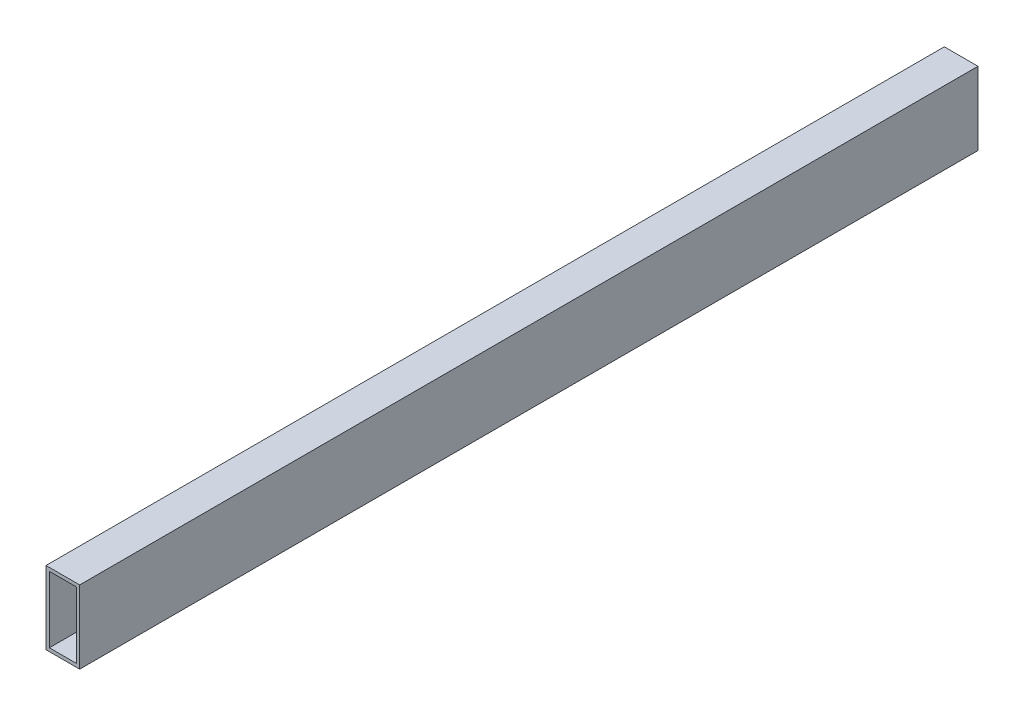
SolidWorks part; units mm, degrees
material "不锈钢管"
ref_plane "Front Plane" through (0, 0, 0) normal (0, 0, 1) x (1, 0, 0)
ref_plane "Top Plane" through (0, 0, 0) normal (0, 1, 0) x (1, 0, 0)
ref_plane "Right Plane" through (0, 0, 0) normal (1, 0, 0) x (0, 0, -1)
other "Configuration Table"
sketch "Sketch1" plane through (0, 0, 0) normal (0, 0, 1) x (1, 0, 0)
  line L0 (-40.8525, 38.9734) -> (-40.8525, -26.0266)
  line L1 (-40.8525, -26.0266) -> (-10.8525, -26.0266)
  line L2 (-10.8525, -26.0266) -> (-10.8525, 38.9734)
  line L3 (-10.8525, 38.9734) -> (-40.8525, 38.9734)
  dimension "D1" = 30
  dimension "D2" = 65
extrude "Boss-Extrude1" add sketch "Sketch1" along normal blind 800
sketch "Sketch2" plane through (0, 0, 800) normal (0, 0, 1) x (1, 0, 0)
  line L0 (-37.8525, 35.2071) -> (-37.8525, -23.0266)
  line L1 (-37.8525, -23.0266) -> (-13.8525, -23.0266)
  line L2 (-13.8525, -23.0266) -> (-13.8525, 35.9734)
  line L3 (-13.8525, 35.9734) -> (-37.8525, 35.9734)
  line L4 (-10.8525, -26.0266) -> (-10.8525, 38.9734) construction
  line L5 (-40.8525, -26.0266) -> (-10.8525, -26.0266) construction
  line L6 (-40.8525, 38.9734) -> (-40.8525, -26.0266) construction
  line L7 (-10.8525, 38.9734) -> (-40.8525, 38.9734) construction
  line L8 (-37.8525, 35.2071) -> (-37.8525, 35.9734)
  dimension "D1" = 3
  dimension "D2" = 3
  dimension "D3" = 3
  dimension "D4" = 3
extrude "Cut-Extrude1" cut sketch "Sketch2" against normal blind 800
sketch "Sketch3" plane through (-10.8525, 0, 0) normal (1, 0, 0) x (0, 0, -1)
  circle A0 centre (-748.9135, 6.4734) radius 17.2688
